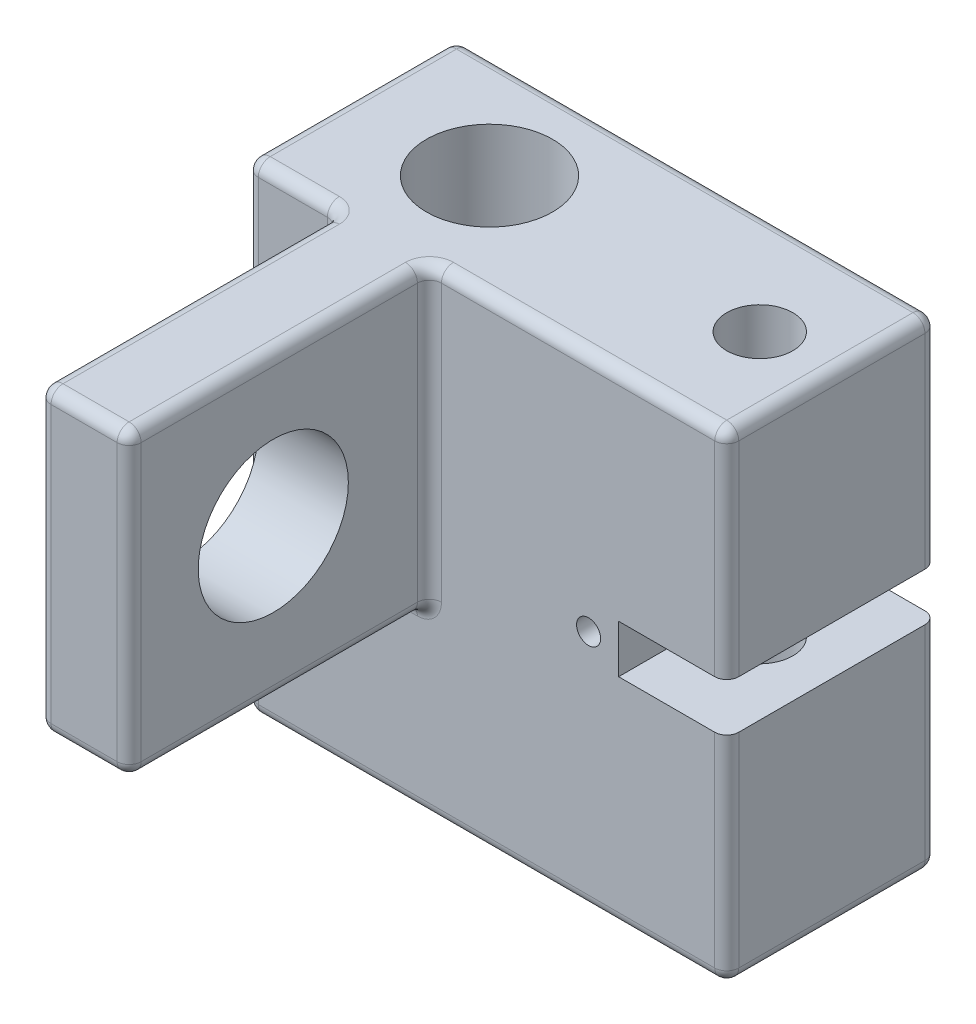
SolidWorks part; units mm, degrees
material "Beech"
ref_plane "Front Plane" through (0, 0, 0) normal (0, 0, 1) x (1, 0, 0)
ref_plane "Top Plane" through (0, 0, 0) normal (0, 1, 0) x (1, 0, 0)
ref_plane "Right Plane" through (0, 0, 0) normal (1, 0, 0) x (0, 0, -1)
sketch "Sketch1" plane through (0, 0, 0) normal (0, 1, 0) x (1, 0, 0)
  line L0 (23, 0) -> (23, 90.8533) construction
  line L1 (0, 0) -> (80, 0)
  line L2 (0, 0) -> (0, 35)
  line L3 (0, 35) -> (80, 35)
  line L4 (80, 0) -> (80, 35)
  line L6 (30.5, 0) -> (15.5, 0)
  line L7 (30.5, 0) -> (30.5, -50)
  line L8 (30.5, -50) -> (15.5, -50)
  line L9 (15.5, 0) -> (15.5, -50)
  circle A0 centre (68, 17.5) radius 5.5
  circle A1 centre (23, 17.5) radius 10.5
  dimension "D3" = 45
  dimension "D4" = 11
  dimension "D5" = 21
  dimension "D6" = 17.5
  dimension "D7" = 12
  dimension "D1" = 80
  dimension "D2" = 35
  dimension "D8" = 15
  dimension "D9" = 50
extrude "Boss-Extrude1" add sketch "Sketch1" along normal mid plane 80 contours L1 L0 A1 L3 L2 | L0 L1 L4 L3 L6 A1 A0 | L0 L6 L9 L8
sketch "Sketch2" plane through (0, 0, 0) normal (-1, 0, 0) x (0, 0, 1)
  line L0 (0, 0) -> (-45.2738, 0) construction
  line L1 (0, 40) -> (0, -40) construction
  circle A0 centre (-17.5, 22.5) radius 6
  circle A1 centre (-17.5, -22.5) radius 6
  dimension "D1" = 12
  dimension "D2" = 45
  dimension "D3" = 17.5
extrude "Cut-Extrude1" cut sketch "Sketch2" against normal blind 10
sketch "Sketch4" plane through (30.5, 0, 0) normal (1, 0, 0) x (0, 0, -1)
  line L0 (0, -40) -> (-50, -40) construction
  line L1 (-50, -40) -> (0, -40)
  line L2 (-50, -40) -> (-50, -10)
  line L3 (-50, -10) -> (0, -10)
  line L4 (0, -40) -> (0, -10)
  line L6 (0, 40) -> (-50, 40) construction
  line L7 (0, 40) -> (0, -40) construction
  dimension "D1" = 50
extrude "Cut-Extrude3" cut sketch "Sketch4" against normal through all
sketch "Sketch3" plane through (30.5, 0, 0) normal (1, 0, 0) x (0, 0, -1)
  line L0 (0, 40) -> (-50, 40) construction
  line L1 (0, 40) -> (0, -10) construction
  circle A0 centre (-26, 15) radius 12.5
  dimension "D1" = 26
  dimension "D2" = 25
  dimension "D3" = 25
extrude "Cut-Extrude2" cut sketch "Sketch3" against normal blind 15
sketch "Sketch6" plane through (0, 0, 0) normal (0, 0, 1) x (1, 0, 0)
  line L0 (80, 40) -> (80, -40) construction
  line L1 (80, 4) -> (62, 4)
  line L2 (80, 4) -> (80, -4)
  line L3 (80, -4) -> (62, -4)
  line L4 (62, 4) -> (62, -4)
  line L5 (0, 0) -> (83.9174, 0) construction
  dimension "D1" = 8
  dimension "D2" = 18
extrude "Cut-Extrude4" cut sketch "Sketch6" against normal through all
fillet "Fillet1" radius 2 26 edges at (55.25, 40, 0) (40, -40, 0) (0, -40, -17.5) (40, -40, -35) (80, 40, -17.5) (80, -40, -17.5) (40, 40, -35) (30.5, 15, 50) (15.5, 15, 50) (15.5, 15, 0) (0, 0, 0) (0, 0, -35) (80, 22, -35) (80, 22, 0) (30.5, 15, 0) (0, 40, -17.5) (7.75, 40, 0) (15.5, 40, 25) (23, 40, 50) (15.5, -10, 25) (23, -10, 50) (23, -10, 0) (30.5, -10, 25) (30.5, 40, 25) (80, -22, 0) (80, -22, -35)
sketch "Sketch7" plane through (0, 0, 0) normal (0, 0, 1) x (1, 0, 0)
  line L1 (62, 4) -> (62, -4) construction
  circle A0 centre (57, 0) radius 2
  dimension "D1" = 4
  dimension "D2" = 5
extrude "Cut-Extrude5" cut sketch "Sketch7" against normal through all
